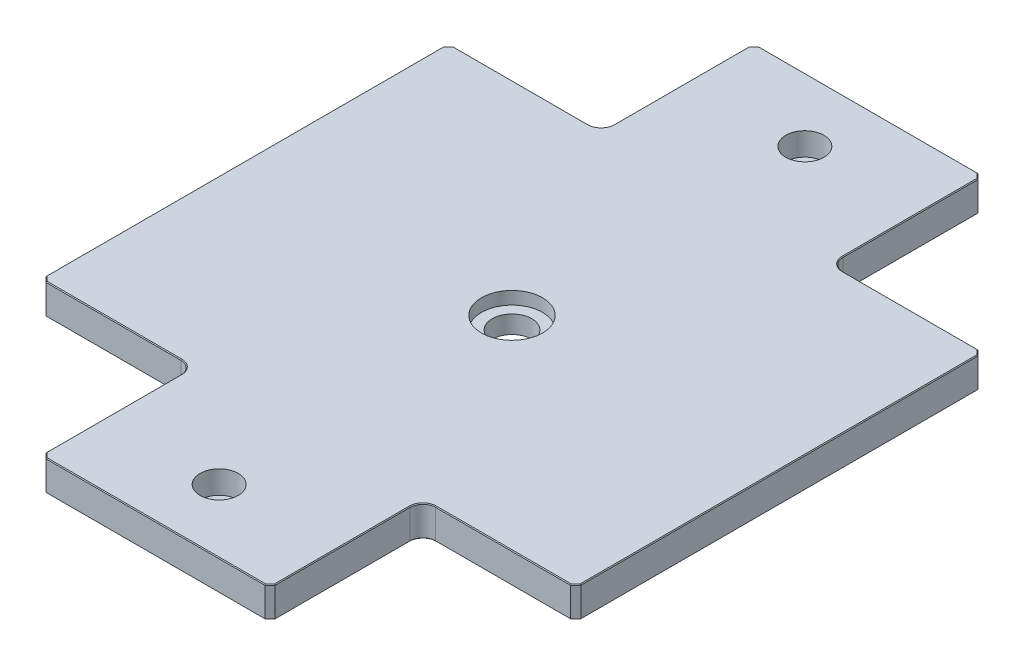
SolidWorks part; units mm, degrees
material "Al6061"
ref_plane "Front" through (0, 0, 0) normal (0, 0, 1) x (1, 0, 0)
ref_plane "Top" through (0, 0, 0) normal (0, 1, 0) x (1, 0, 0)
ref_plane "Right" through (0, 0, 0) normal (1, 0, 0) x (0, 0, -1)
sketch "草图1" plane through (0, 0, 0) normal (0, 1, 0) x (1, 0, 0)
  line L0 (-105, 140) -> (105, -140) construction
  line L1 (-105, -140) -> (105, -140)
  line L2 (-105, -140) -> (-105, 140)
  line L3 (-105, 140) -> (105, 140)
  line L4 (105, -140) -> (105, 140)
  dimension "D1" = 280
  dimension "D2" = 210
extrude "凸台-拉伸1" add sketch "草图1" along normal blind 12
sketch "草图2" plane through (0, 12, 0) normal (0, 1, 0) x (1, 0, 0)
  line L0 (0, -115) -> (0, 115) construction
  circle A0 centre (0, 0) radius 7.75
  circle A1 centre (0, -115) radius 4.5
  circle A2 centre (0, 115) radius 4.5
  dimension "D1" = 9
  dimension "D3" = 15.5
  dimension "D2" = 230
extrude "切除-拉伸1" cut sketch "草图2" against normal through all
sketch "草图3" plane through (0, 12, 0) normal (0, 1, 0) x (1, 0, 0)
  line L1 (-105, -140) -> (-45, -140)
  line L2 (-105, -140) -> (-105, -80)
  line L3 (-105, -80) -> (-45, -80)
  line L4 (-45, -140) -> (-45, -80)
  line L5 (-105, 140) -> (-45, 140)
  line L6 (-105, 140) -> (-105, 80)
  line L7 (-105, 80) -> (-45, 80)
  line L8 (-45, 140) -> (-45, 80)
  line L9 (105, 140) -> (45, 140)
  line L10 (105, 140) -> (105, 80)
  line L11 (105, 80) -> (45, 80)
  line L12 (45, 140) -> (45, 80)
  line L13 (105, -140) -> (45, -140)
  line L14 (105, -140) -> (105, -80)
  line L15 (105, -80) -> (45, -80)
  line L16 (45, -140) -> (45, -80)
  dimension "D1" = 60
extrude "切除-拉伸2" cut sketch "草图3" against normal through all
fillet "圆角1" radius 5 4 edges at (-45, 6, -80) (45, 6, -80) (45, 6, 80) (-45, 6, 80)
chamfer "倒角1" distance 2 angle 45 8 edges at (105, 6, 80) (45, 6, 140) (-45, 6, 140) (-105, 6, 80) (-105, 6, -80) (-45, 6, -140) (105, 6, -80) (45, 6, -140)
sketch "草图4" plane through (0, 12, 0) normal (0, 1, 0) x (1, 0, 0)
  circle A0 centre (0, -115) radius 7.5
  circle A1 centre (0, 115) radius 7.5
  dimension "D1" = 15
extrude "切除-拉伸3" cut sketch "草图4" against normal blind 9
sketch "草图5" plane through (0, 12, 0) normal (0, 1, 0) x (1, 0, 0)
  circle A0 centre (0, 0) radius 12
  dimension "D1" = 24
extrude "切除-拉伸4" cut sketch "草图5" against normal blind 5
chamfer "倒角2" distance 0.3 angle 45 24 edges at (-76.5, 12, 80) (-46.4645, 12, 81.4645) (-45, 12, 111.5) (-44, 12, 139) (0, 12, 140) (44, 12, 139) (45, 12, 111.5) (46.4645, 12, 81.4645) (76.5, 12, 80) (104, 12, 79) (105, 12, 0) (104, 12, -79) (76.5, 12, -80) (46.4645, 12, -81.4645) (45, 12, -111.5) (44, 12, -139) (0, 12, -140) (-44, 12, -139) (-45, 12, -111.5) (-46.4645, 12, -81.4645) (-104, 12, 79) (-105, 12, 0) (-104, 12, -79) (-76.5, 12, -80)
chamfer "倒角3" distance 0.3 angle 45 24 edges at (-44, 0, -139) (0, 0, -140) (44, 0, -139) (45, 0, -111.5) (46.4645, 0, -81.4645) (76.5, 0, -80) (104, 0, -79) (105, 0, 0) (104, 0, 79) (76.5, 0, 80) (46.4645, 0, 81.4645) (45, 0, 111.5) (44, 0, 139) (0, 0, 140) (-44, 0, 139) (-45, 0, 111.5) (-45, 0, -111.5) (-46.4645, 0, 81.4645) (-46.4645, 0, -81.4645) (-76.5, 0, 80) (-104, 0, 79) (-105, 0, 0) (-104, 0, -79) (-76.5, 0, -80)
